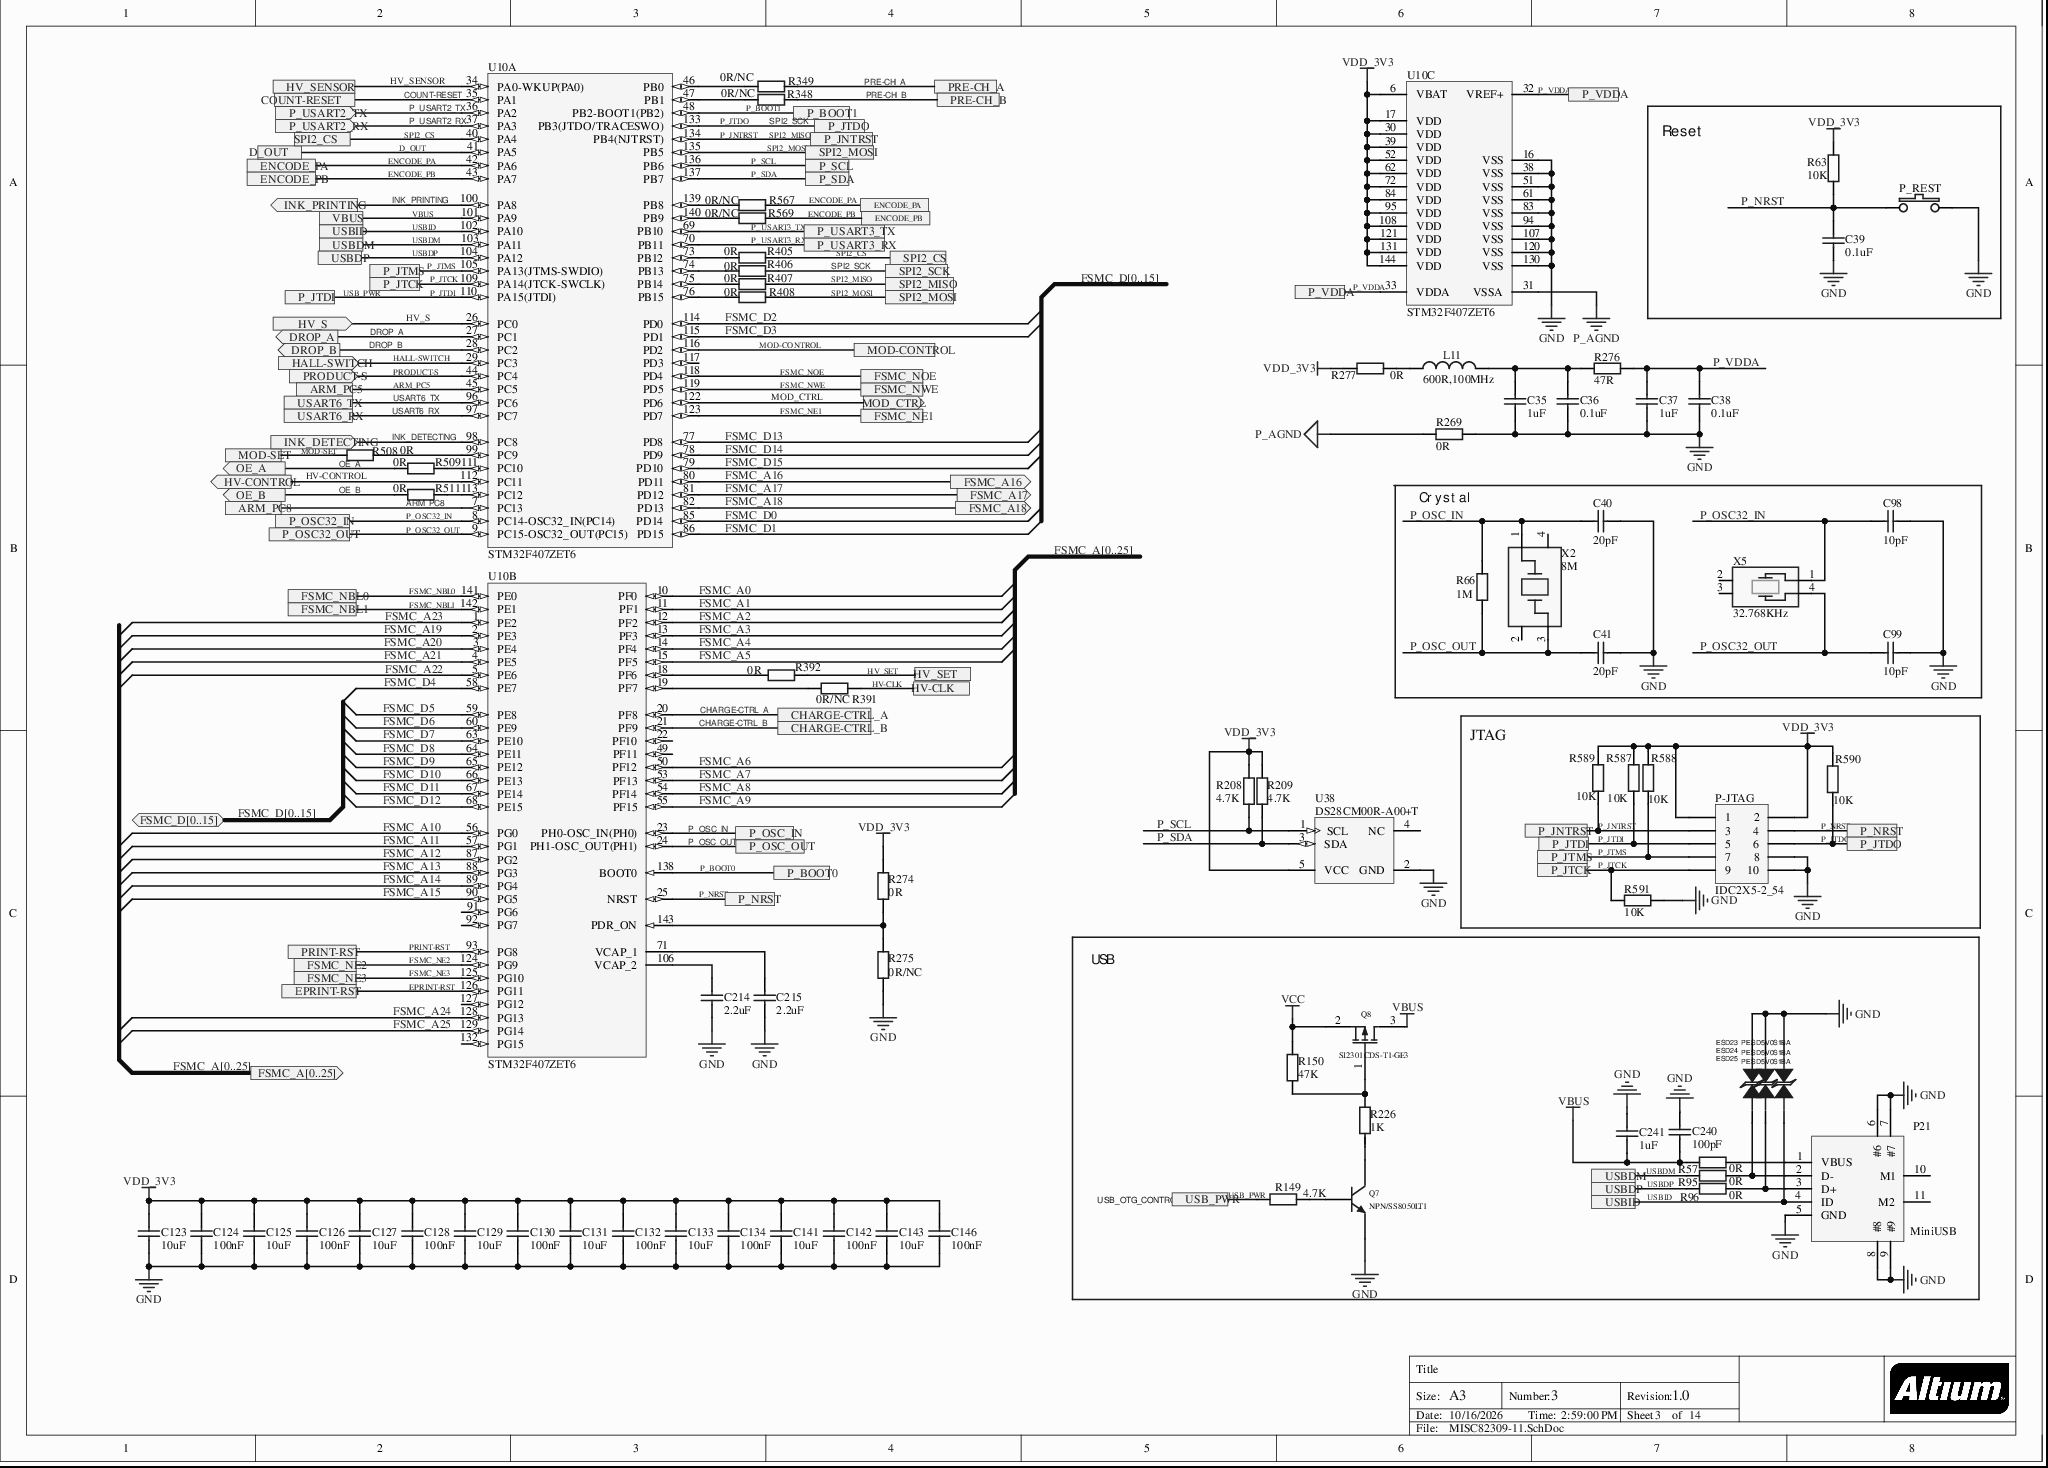
[diagram p0: MISC82309-11.SchDoc]
# Altium project MISC82309-16.PrjPcb (part 2 of 6)
## Sheet MISC82309-11.SchDoc (continued)
### Nets (continued)
ARM_PC5: U10.45(PC5) ; port ARM_PC5
ARM_PC8: U10.7(PC13) ; port ARM_PC8
CHARGE-CTRL_A: U10.20(PF8) ; port CHARGE-CTRL_A
CHARGE-CTRL_B: U10.21(PF9) ; port CHARGE-CTRL_B
COUNT-RESET: U10.35(PA1) ; port COUNT-RESET
D_OUT: U10.41(PA5) ; port D_OUT
DROP_A: U10.27(PC1) ; port DROP_A
DROP_B: U10.28(PC2) ; port DROP_B
ENCODE_PA: R567.2 U10.42(PA6) ; port ENCODE_PA
ENCODE_PB: R569.2 U10.43(PA7) ; port ENCODE_PB
EPRINT-RST: U10.126(PG11) ; port EPRINT-RST
FSMC_A0: U10.10(PF0)
FSMC_A1: U10.11(PF1)
FSMC_A2: U10.12(PF2)
FSMC_A3: U10.13(PF3)
FSMC_A4: U10.14(PF4)
FSMC_A5: U10.15(PF5)
FSMC_A6: U10.50(PF12)
FSMC_A7: U10.53(PF13)
FSMC_A8: U10.54(PF14)
FSMC_A9: U10.55(PF15)
FSMC_A10: U10.56(PG0)
FSMC_A11: U10.57(PG1)
FSMC_A12: U10.87(PG2)
FSMC_A13: U10.88(PG3)
FSMC_A14: U10.89(PG4)
FSMC_A15: U10.90(PG5)
FSMC_A16: U10.80(PD11) ; port FSMC_A16
FSMC_A17: U10.81(PD12) ; port FSMC_A17
FSMC_A18: U10.82(PD13) ; port FSMC_A18
FSMC_A19: U10.2(PE3)
FSMC_A20: U10.3(PE4)
FSMC_A21: U10.4(PE5)
FSMC_A22: U10.5(PE6)
FSMC_A23: U10.1(PE2)
FSMC_A24: U10.128(PG13)
FSMC_A25: U10.129(PG14)
FSMC_D0: U10.85(PD14)
FSMC_D1: U10.86(PD15)
FSMC_D2: U10.114(PD0)
FSMC_D3: U10.115(PD1)
FSMC_D4: U10.58(PE7)
FSMC_D5: U10.59(PE8)
FSMC_D6: U10.60(PE9)
FSMC_D7: U10.63(PE10)
FSMC_D8: U10.64(PE11)
FSMC_D9: U10.65(PE12)
FSMC_D10: U10.66(PE13)
FSMC_D11: U10.67(PE14)
FSMC_D12: U10.68(PE15)
FSMC_D13: U10.77(PD8)
FSMC_D14: U10.78(PD9)
FSMC_D15: U10.79(PD10)
FSMC_NBL0: U10.141(PE0) ; port FSMC_NBL0
FSMC_NBL1: U10.142(PE1) ; port FSMC_NBL1
FSMC_NE1: U10.123(PD7) ; port FSMC_NE1
FSMC_NE2: U10.124(PG9) ; port FSMC_NE2
FSMC_NE3: U10.125(PG10) ; port FSMC_NE3
FSMC_NOE: U10.118(PD4) ; port FSMC_NOE
FSMC_NWE: U10.119(PD5) ; port FSMC_NWE
HALL-SWITCH: U10.29(PC3) ; port HALL-SWITCH
HV-CLK: R391.2 ; port HV-CLK
HV-CONTROL: U10.112(PC11) ; port HV-CONTROL
HV_S: U10.26(PC0) ; port HV_S
HV_SENSOR: U10.34(PA0-WKUP(PA0)) ; port HV_SENSOR
HV_SET: R392.2 ; port HV_SET
INK_DETECTING: U10.98(PC8) ; port INK_DETECTING
INK_PRINTING: U10.100(PA8) ; port INK_PRINTING
MOD-CONTROL: U10.116(PD2) ; port MOD-CONTROL
MOD-SET: R508.2 ; port MOD-SET
MOD_CTRL: U10.122(PD6) ; port MOD_CTRL
OE_A: R509.1 ; port OE_A
OE_B: R511.1 ; port OE_B
P_BOOT0: U10.138(BOOT0) ; port P_BOOT0
P_BOOT1: U10.48(PB2-BOOT1(PB2)) ; port P_BOOT1
P_JNTRST: P-JTAG.3 R407.2 R589.1 U10.134(PB4(NJTRST)) ; port P_JNTRST, port SPI2_MISO  [also labelled SPI2_MISO]
P_JTCK: P-JTAG.9 R591.2 U10.109(PA14(JTCK-SWCLK)) ; port P_JTCK
P_JTDI: P-JTAG.5 R149.1 R587.1 U10.110(PA15(JTDI)) ; port USB_PWR, port P_JTDI  [also labelled USB_PWR]
P_JTDO: P-JTAG.6 R406.2 R590.1 U10.133(PB3(JTDO/TRACESWO)) ; port P_JTDO, port SPI2_SCK  [also labelled SPI2_SCK]
P_JTMS: P-JTAG.7 R588.1 U10.105(PA13(JTMS-SWDIO)) ; port P_JTMS
P_NRST: C39.2 P-JTAG.4 P_REST.1 R63.2 U10.25(NRST) ; port P_NRST
P_OSC32_IN: C98.2 U10.8(PC14-OSC32_IN(PC14)) X5.1 ; port P_OSC32_IN
P_OSC32_OUT: C99.2 U10.9(PC15-OSC32_OUT(PC15)) X5.4 ; port P_OSC32_OUT
P_OSC_IN: C40.2 R66.1 U10.23(PH0-OSC_IN(PH0)) X2.1 ; port P_OSC_IN
P_OSC_OUT: C41.2 R66.2 U10.24(PH1-OSC_OUT(PH1)) X2.3 ; port P_OSC_OUT
P_SCL: R208.2 U10.136(PB6) U38.1(SCL) ; port P_SCL
P_SDA: R209.2 U10.137(PB7) U38.3(SDA) ; port P_SDA
P_USART2_RX: U10.37(PA3) ; port P_USART2_RX
P_USART2_TX: U10.36(PA2) ; port P_USART2_TX
P_USART3_RX: U10.70(PB11) ; port P_USART3_RX
P_USART3_TX: U10.69(PB10) ; port P_USART3_TX
P_VDDA: C37.2 C38.2 R276.2 U10.32(VREF+) U10.33(VDDA) ; port P_VDDA
PRE-CH_A: R349.2 ; port PRE-CH_A
PRE-CH_B: R348.2 ; port PRE-CH_B
PRINT-RST: U10.93(PG8) ; port PRINT-RST
PRODUCT-S: U10.44(PC4) ; port PRODUCT-S
SPI2_CS: R405.2 U10.40(PA4) ; port SPI2_CS
SPI2_MOSI: R408.2 U10.135(PB5) ; port SPI2_MOSI
USART6_RX: U10.97(PC7) ; port USART6_RX
USART6_TX: U10.96(PC6) ; port USART6_TX
USBDM: R95.2 U10.103(PA11) ; port USBDM
USBDP: R96.2 U10.104(PA12) ; port USBDP
USBID: ESD23.1 P21.4(ID) U10.102(PA10) ; port USBID
NetC35_2: C35.2 C36.2 L11.2 R276.1
NetC214_1: C214.1 U10.106(VCAP_2)
NetC215_1: C215.1 U10.71(VCAP_1)
NetESD24_1: ESD24.1 P21.2(D-) R95.1
NetESD25_1: ESD25.1 P21.3(D+) R96.1
NetL11_1: L11.1 R277.2
NetP21_1: P21.1(VBUS) R57.1
NetQ7_1: Q7.1(B) R149.2
NetQ7_3: Q7.3(C) R226.2
NetQ8_1: Q8.1(G) R150.1 R226.1
NetR274_1: R274.1 R275.2 U10.143(PDR_ON)
NetR348_1: R348.1 U10.47(PB1)
NetR349_1: R349.1 U10.46(PB0)
NetR391_1: R391.1 U10.19(PF7)
NetR392_1: R392.1 U10.18(PF6)
NetR405_1: R405.1 U10.73(PB12)
NetR406_1: R406.1 U10.74(PB13)
NetR407_1: R407.1 U10.75(PB14)
NetR408_1: R408.1 U10.76(PB15)
NetR508_1: R508.1 U10.99(PC9)
NetR509_2: R509.2 U10.111(PC10)
NetR511_2: R511.2 U10.113(PC12)
NetR567_1: R567.1 U10.139(PB8)
NetR569_1: R569.1 U10.140(PB9)

Not connected (* = marked no-connect by the designer): P21 10(M1) 11(M2); P_REST 5 6; U10 22(PF10) 49(PF11) 91(PG6) 92(PG7) 117(PD3) 127(PG12) 132(PG15); U38 4(NC); X2 2 4; X5 2 3

### Buses and harness runs
bus FSMC_A[0..25]
bus FSMC_A[0..25] = port FSMC_A[0..25]
bus FSMC_D[0..15]
bus FSMC_D[0..15] = port FSMC_D[0..15]

### Notes on the sheet
- USB_OTG_CONTROL
- Title
- Size:
- Date:
- A3
- Number:
- Time:
- Revision:
- Sheet
- of
- File:

### Library data of the parts
C35-C38 C214 C215 = CAP_0805: Capacitor
  C35 C37: value: 1uF
  C36 C38: value: 0.1uF
  C214 C215: value: 2.2uF
C39 = CAP_1206: Capacitor; value: 0.1uF
C40 C41 C98 C99 C123-C134 C141-C143 C146 = CAP_1206: Capacitor; value: 0.1uF
C240 C241 = CAP_0603: Capacitor
  C240: value: 100pF
  C241: value: 1uF
ESD23-ESD25 = DIODE_TVS_BI-DIR: TVS,BIDIRECTION,5V,RENESAS PROJECT; Manufacturer: NXP; Part_Number: ESDEMI44; SMT_OPTION: YES; Lib_from: MIKE; PACKAGE: SOD882; Manufacturer_Part_Number: PESD5V0S1BA; Description_2: TVS,BIDIRECTION,5V,RENESAS PROJECT; PCB DECAL: SOD323
L11 = Inductor: value: 600R,100MHz
P21 = USB_Slave
P-JTAG = HEAD2X5-2_54
Q7 = NPN: YFLZVQMB: MB4A050S1; AIEP: 43; NRXQ: Transistor; GGULWYUT: SMD NPN transistor, 1.5A, 25V, 0.3W, Ft=100MHZ, Hfe range 120-350; BSHU: SOT-23; ZJYF: PCS; TQWQXLGC: Sunlord; DWCHAXEP: SS8050LT1; PCB DECAL: SOT-23-3; Value: NPN/SS8050LT1; Comment_1: NPN
Q8 = SI2301: MOSFET; YFLZVQMB: MB4E23010; GGULWYUT: SMD PMOS, -20V,-3.1A,1.6W, on-resistance 112mΩ, Qg typical 3.3nC; TQWQXLTW: VISAY; DWCHAXEP: SI2301CDS-T1-GE3; YQWWAXEP: *; PCB DECAL: SOT-23; Comment_1: SI2301
R57 R95 R96 R150 R226 R274 R275 R348 R349 R391 R392 R405-R408 R508 R509 R511 R567 R569 = Res_0603: Res
  R57 R95 R96 R274 R392 R405-R408 R508 R509 R511: value: 0R
  R150: value: 47K
  R226: value: 1K
  R275 R348 R349 R391 R567 R569: value: 0R/NC
R63 R208 R209 = Res2: Resistor; Published: 8-Jun-2000; LatestRevisionDate: 17-Jul-2002; LatestRevisionNote: Re-released for DXP Platform.; PackageReference: AXIAL-0.4; Publisher: Altium Limited
  R63: Value: 10K
  R208 R209: Value: 4.7K
R66 = Res2: Resistor; Value: 10K; Published: 8-Jun-2000; LatestRevisionDate: 17-Jul-2002; LatestRevisionNote: Re-released for DXP Platform.; PackageReference: AXIAL-0.4; Publisher: Altium Limited
R149 = Res2: Resistor; Value: 1K; Published: 8-Jun-2000; LatestRevisionDate: 17-Jul-2002; LatestRevisionNote: Re-released for DXP Platform.; PackageReference: AXIAL-0.4; Publisher: Altium Limited
R269 R276 R277 = Res_0805: Res
  R269 R277: value: 0R
  R276: value: 47R
R587-R591 = Res: value: 10K
U10 = STM32F407ZET6: ARM Cortex-M4 32-bit MCU+FPU, 210 DMIPS, 512 kB Flash, 192 kB Internal RAM, 114 I/Os, 144-pin LQFP, -40 to 85 degC, Tray; Manufacturer: STMicroelectronics; D/A Converter: 2x12-bit; FLASH Size (Prog) (kB): 512; I/Os (High Current): 114; Internal RAM Size (kB): 192; Operating Frequency(F) (Processor speed) (MHz): 168; Supply Voltage(Vcc) max (V): 3.6; Supply Voltage(Vcc) min (V): 1.8; DatasheetVersion: Rev. 4; PackageVersion: Rev. 4, 06/2013; PackageReference: LQFP144; PackageDescription: 144-Pin Low Profile Quad Flat Package, 20 x 20 mm Body, 0.5 mm Pitch; Supplier 1: Digi-Key; Supplier Part Number 1: 497-11903-ND; Supplier 2: Farnell; Supplier Part Number 2: 2215229; Supplier 3: Newark; Supplier Part Number 3: 46W2203; Supplier 4: Newark; Supplier Part Number 4: 87T3795; Supplier 5: Mouser; Supplier Part Number 5: 511-STM32F407ZET6; Core: ARM Cortex-M4; Packing: Tray; Mounting Technology: Surface Mount; PartNumber: STM32F407ZET6; ComponentLink1Description: Manufacturer URL; ComponentLink1URL: http://www.st.com/web/en/home.html; ComponentLink2Description: Datasheet; ComponentLink2URL: http://www.st.com/st-web-ui/static/active/en/resource/technical/document/datasheet/DM00037051.pdf; ComponentLink3Description: Package Specification; ComponentLink3URL: http://www.st.com/st-web-ui/static/active/en/resource/technical/document/datasheet/DM00037051.pdf
U38 = DS28CM00R-A00+T: I睠/SMBus Silicon Serial Number, 5-pin SOT23, -40?to + 85?C, Pb-Free, Tape and Reel; DatasheetVersion: 1/11/2006; PackageVersion: revF, 2006; PackageReference: U5+1; PackageDescription: 5-Pin Small-Outline Transistor Package, 0.95 mm Pitch, 2.8 mm Lead Span, SOT-23, Pb-Free; Code_JEDEC: MO-178AA; ComponentLink1Description: Manufacturer URL; ComponentLink1URL: www.maxim-ic.com; ComponentLink2Description: Datasheet; ComponentLink2URL: http://datasheets.maxim-ic.com/en/ds/DS28CM00.pdf
X2 = CRYSTAL-SMD4: value: SMD5032_8MHZ_4pin
X5 = CRYSTAL-SMD4A: value: 晶体SSP-T7-F32.768KHZ

## Sheet MISC82309-10.SchDoc
size A3; DocumentNumber: 4; Revision: 1.0; SheetNumber: 4; SheetTotal: 14
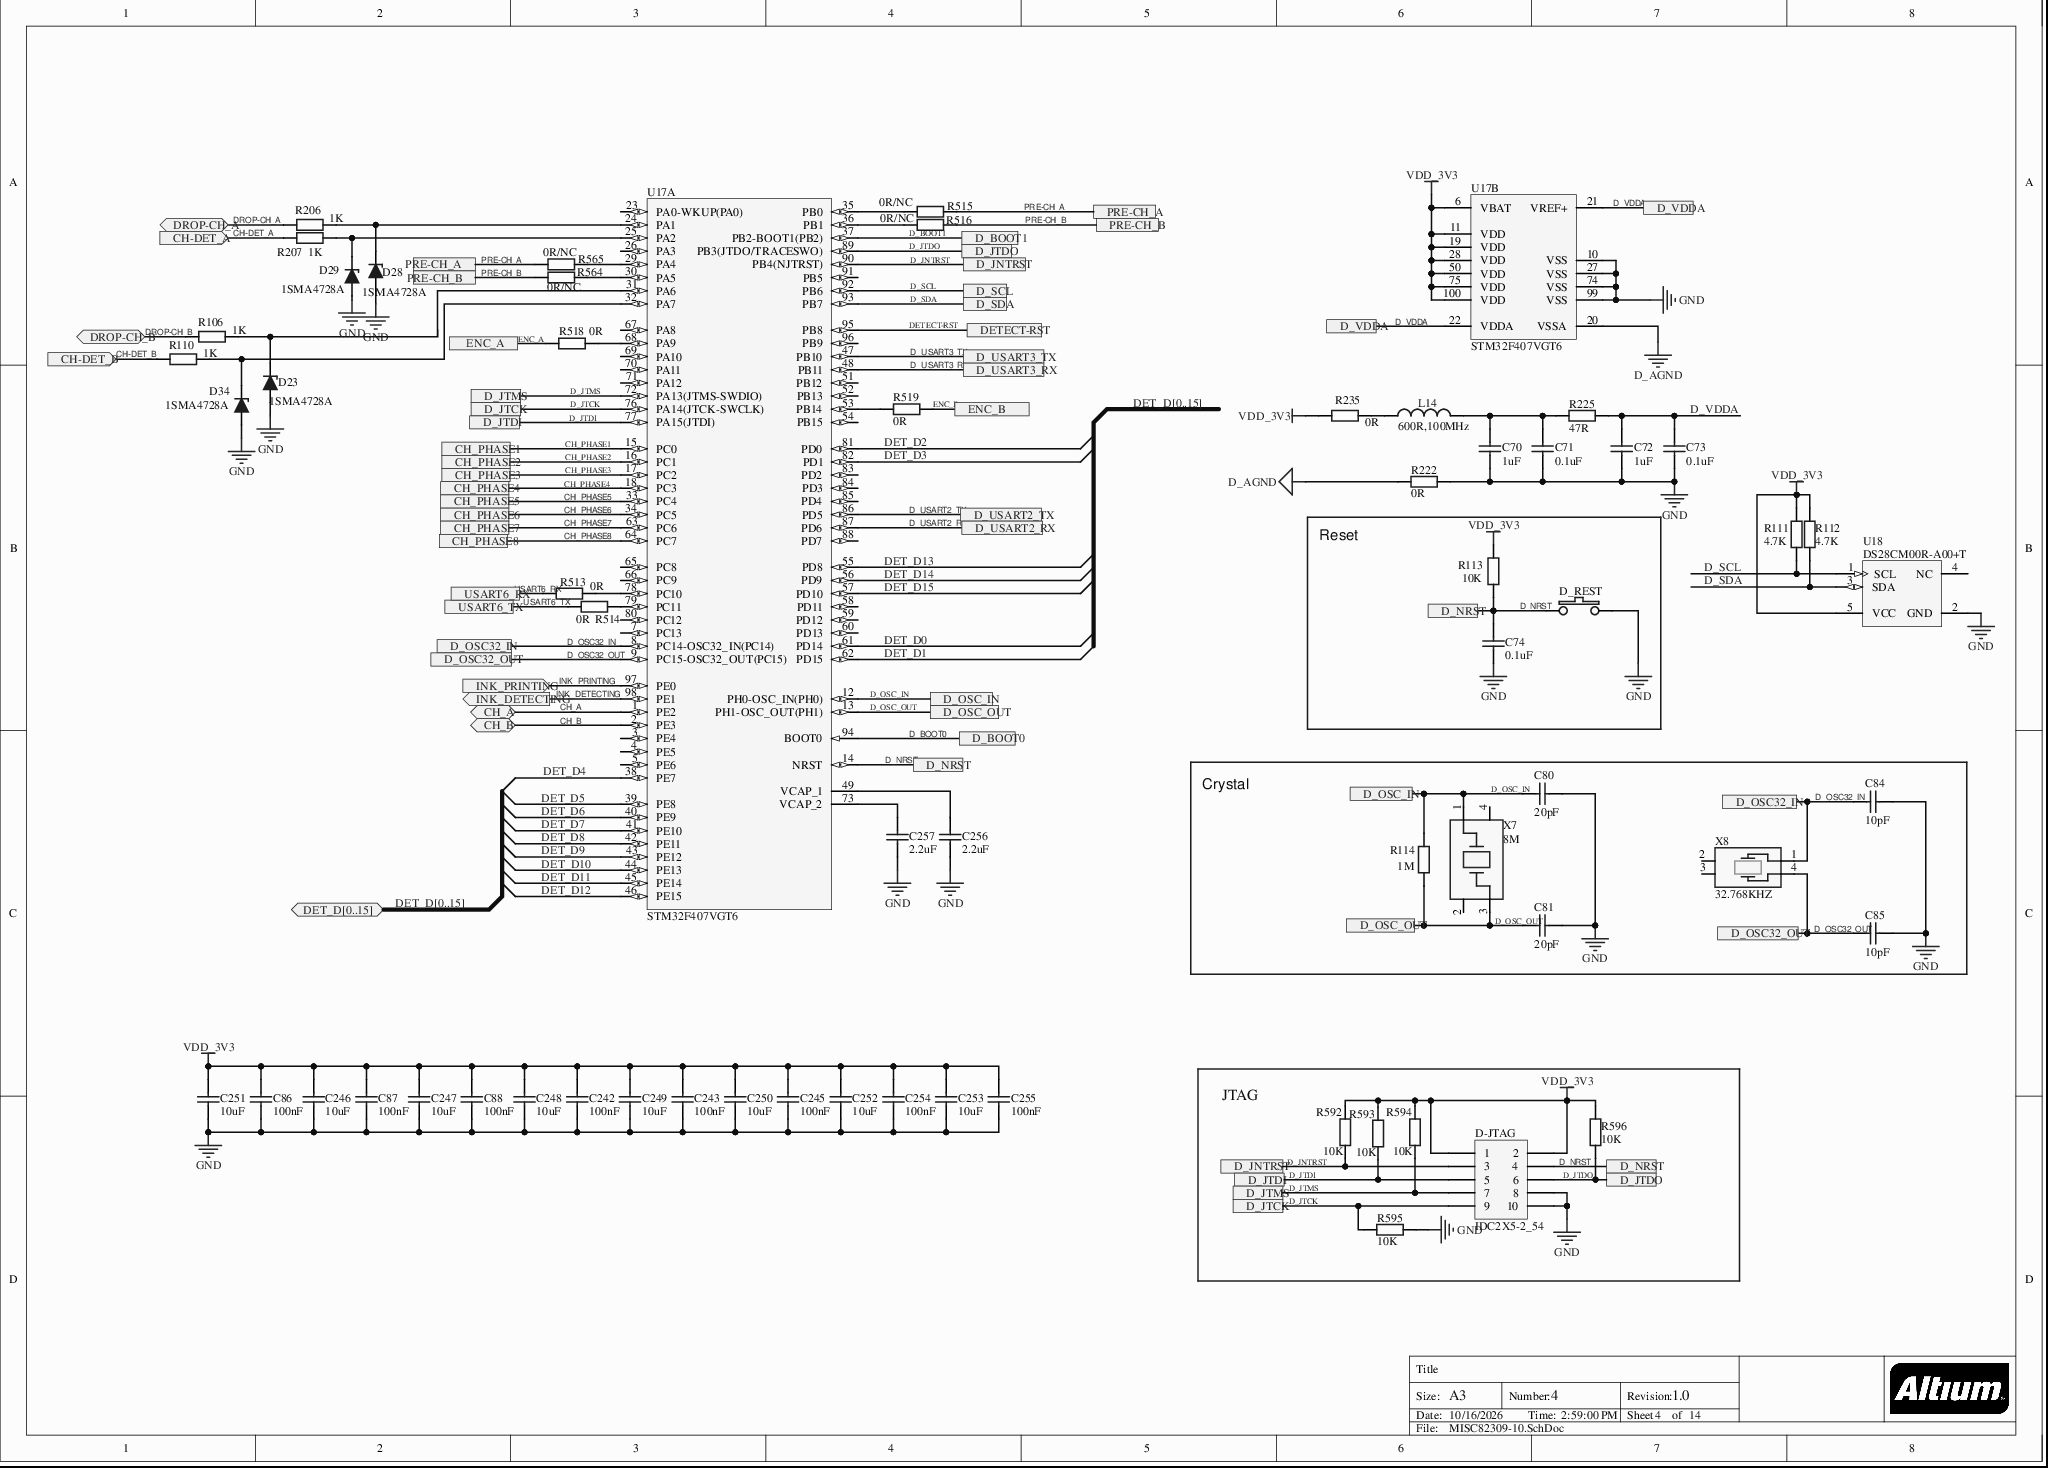
[diagram p1: MISC82309-10.SchDoc]

### Parts
C70  1uF  [CAP_0805]
C71  0.1uF  [CAP_0805]
C72  1uF  [CAP_0805]
C73  0.1uF  [CAP_0805]
C74  0.1uF  [C0603]
C80  20pF  [C0603]
C81  20pF  [C0603]
C84  10pF  [C0603]
C85  10pF  [C0603]
C86  100nF  [C0805]
C87  100nF  [C0805]
C88  100nF  [C0805]
C242  100nF  [C0805]
C243  100nF  [C0805]
C245  100nF  [C0805]
C246  10uF  [C0805]
C247  10uF  [C0805]
C248  10uF  [C0805]
C249  10uF  [C0805]
C250  10uF  [C0805]
C251  10uF  [C0805]
C252  10uF  [C0805]
C253  10uF  [C0805]
C254  100nF  [C0805]
C255  100nF  [C0805]
C256  2.2uF  [CAP_0805]
C257  2.2uF  [CAP_0805]
D23  1SMA4728A  [DO-214AC]
D28  1SMA4728A  [DO-214AC]
D29  1SMA4728A  [DO-214AC]
D34  1SMA4728A  [DO-214AC]
D-JTAG  IDC2X5-2_54  [IDC2X5-2_54]
D_REST  SW  [SW-6X3X2.5]  (value not drawn)
L14  600R,100MHz  [R0805]
R106  1K  [R1206]
R110  1K  [R1206]
R111  4.7K  [R0603]
R112  4.7K  [R0603]
R113  10K  [R0603]
R114  1M  [R0603]
R206  1K  [R1206]
R207  1K  [R1206]
R222  0R  [R0805]
R225  47R  [R0805]
R235  0R  [R0805]
R513  0R  [RES_0603]
R514  0R  [RES_0603]
R515  0R/NC  [RES_0603]
R516  0R/NC  [RES_0603]
R518  0R  [RES_0603]
R519  0R  [RES_0603]
R564  0R/NC  [RES_0603]
R565  0R/NC  [RES_0603]
R592  10K  [R0603]
R593  10K  [R0603]
R594  10K  [R0603]
R595  10K  [R0603]
R596  10K  [R0603]
U17  STM32F407VGT6  [LQFP100_N]  (parts A,B of 2)
U18  DS28CM00R-A00+T  [U5+1_N]
X7  8M  [SMD5032]
X8  32.768KHZ  [Y_XTAL_T7]

### Blocks framed on the sheet
Reset: C74 D_REST R113
Crystal: C80 C81 C84 C85 R114 X7 X8
JTAG: D-JTAG R592-R596

### Ports
CH-DET_A (in), CH-DET_B (in), CH_A (bidir), CH_B (bidir), CH_PHASE1, CH_PHASE2, CH_PHASE3, CH_PHASE4, CH_PHASE5, CH_PHASE6, CH_PHASE7, CH_PHASE8, D_BOOT0, D_BOOT1, D_JNTRST, D_JTCK, D_JTDI, D_JTDO, D_JTMS, D_NRST, D_OSC32_IN, D_OSC32_OUT, D_OSC_IN, D_OSC_OUT, D_SCL, D_SDA, D_USART2_RX, D_USART2_TX, D_USART3_RX, D_USART3_TX, D_VDDA, DET_D[0..15] (bidir), DETECT-RST, DROP-CH_A (bidir), DROP-CH_B (bidir), ENC_A, ENC_B, INK_DETECTING (out), INK_PRINTING (in), PRE-CH_A, PRE-CH_B, USART6_RX, USART6_TX

### Nets
D_AGND: R222.1 U17.20(VSSA)
GND: C70.1 C71.1 C72.1 C73.1 C74.1 C80.1 C81.1 C84.1 C85.1 C86.1 C87.1 C88.1 C242.1 C243.1 C245.1 C246.1 C247.1 C248.1 C249.1 C250.1 C251.1 C252.1 C253.1 C254.1 C255.1 C256.2 C257.2 D23.1 D28.1 D29.1 D34.1 D-JTAG.8 D-JTAG.10 D_REST.2 R222.2 R595.1 U17.10(VSS) U17.27(VSS) U17.74(VSS) U17.99(VSS) U18.2(GND)
VDD_3V3: C86.2 C87.2 C88.2 C242.2 C243.2 C245.2 C246.2 C247.2 C248.2 C249.2 C250.2 C251.2 C252.2 C253.2 C254.2 C255.2 D-JTAG.1 D-JTAG.2 R111.1 R112.1 R113.1 R235.1 R592.2 R593.2 R594.2 R596.1 U17.6(VBAT) U17.11(VDD) U17.19(VDD) U17.28(VDD) U17.50(VDD) U17.75(VDD) U17.100(VDD) U18.5(VCC)
CH-DET_A: R207.1 ; port CH-DET_A
CH-DET_B: R110.1 ; port CH-DET_B
CH_A: U17.1(PE2) ; port CH_A
CH_B: U17.2(PE3) ; port CH_B
CH_PHASE1: U17.15(PC0) ; port CH_PHASE1
CH_PHASE2: U17.16(PC1) ; port CH_PHASE2
CH_PHASE3: U17.17(PC2) ; port CH_PHASE3
CH_PHASE4: U17.18(PC3) ; port CH_PHASE4
CH_PHASE5: U17.33(PC4) ; port CH_PHASE5
CH_PHASE6: U17.34(PC5) ; port CH_PHASE6
CH_PHASE7: U17.63(PC6) ; port CH_PHASE7
CH_PHASE8: U17.64(PC7) ; port CH_PHASE8
D_BOOT0: U17.94(BOOT0) ; port D_BOOT0
D_BOOT1: U17.37(PB2-BOOT1(PB2)) ; port D_BOOT1
D_JNTRST: D-JTAG.3 R592.1 U17.90(PB4(NJTRST)) ; port D_JNTRST
D_JTCK: D-JTAG.9 R595.2 U17.76(PA14(JTCK-SWCLK)) ; port D_JTCK
D_JTDI: D-JTAG.5 R593.1 U17.77(PA15(JTDI)) ; port D_JTDI
D_JTDO: D-JTAG.6 R596.2 U17.89(PB3(JTDO/TRACESWO)) ; port D_JTDO
D_JTMS: D-JTAG.7 R594.1 U17.72(PA13(JTMS-SWDIO)) ; port D_JTMS
D_NRST: C74.2 D-JTAG.4 D_REST.1 R113.2 U17.14(NRST) ; port D_NRST
D_OSC32_IN: C84.2 U17.8(PC14-OSC32_IN(PC14)) X8.1 ; port D_OSC32_IN
D_OSC32_OUT: C85.2 U17.9(PC15-OSC32_OUT(PC15)) X8.4 ; port D_OSC32_OUT
D_OSC_IN: C80.2 R114.1 U17.12(PH0-OSC_IN(PH0)) X7.1 ; port D_OSC_IN
D_OSC_OUT: C81.2 R114.2 U17.13(PH1-OSC_OUT(PH1)) X7.3 ; port D_OSC_OUT
D_SCL: R111.2 U17.92(PB6) U18.1(SCL) ; port D_SCL
D_SDA: R112.2 U17.93(PB7) U18.3(SDA) ; port D_SDA
D_USART2_RX: U17.87(PD6) ; port D_USART2_RX
D_USART2_TX: U17.86(PD5) ; port D_USART2_TX
D_USART3_RX: U17.48(PB11) ; port D_USART3_RX
D_USART3_TX: U17.47(PB10) ; port D_USART3_TX
D_VDDA: C72.2 C73.2 R225.2 U17.21(VREF+) U17.22(VDDA) ; port D_VDDA
DET_D0: U17.61(PD14)
DET_D1: U17.62(PD15)
DET_D2: U17.81(PD0)
DET_D3: U17.82(PD1)
DET_D4: U17.38(PE7)
DET_D5: U17.39(PE8)
DET_D6: U17.40(PE9)
DET_D7: U17.41(PE10)
DET_D8: U17.42(PE11)
DET_D9: U17.43(PE12)
DET_D10: U17.44(PE13)
DET_D11: U17.45(PE14)
DET_D12: U17.46(PE15)
DET_D13: U17.55(PD8)
DET_D14: U17.56(PD9)
DET_D15: U17.57(PD10)
DETECT-RST: U17.95(PB8) ; port DETECT-RST
DROP-CH_A: R206.1 ; port DROP-CH_A
DROP-CH_B: R106.1 ; port DROP-CH_B
ENC_A: R518.2 ; port ENC_A
ENC_B: R519.2 ; port ENC_B
INK_DETECTING: U17.98(PE1) ; port INK_DETECTING
INK_PRINTING: U17.97(PE0) ; port INK_PRINTING
PRE-CH_A: R515.2 R565.1 ; port PRE-CH_A
PRE-CH_B: R516.2 R564.1 ; port PRE-CH_B
USART6_RX: R513.2 ; port USART6_RX
USART6_TX: R514.2 ; port USART6_TX
NetC70_2: C70.2 C71.2 L14.2 R225.1
NetC256_1: C256.1 U17.49(VCAP_1)
NetC257_1: C257.1 U17.73(VCAP_2)
NetD23_2: D23.2 R106.2 U17.31(PA6)
NetD28_2: D28.2 R206.2 U17.24(PA1)
NetD29_2: D29.2 R207.2 U17.25(PA2)
NetD34_2: D34.2 R110.2 U17.32(PA7)
NetL14_1: L14.1 R235.2
NetR513_1: R513.1 U17.78(PC10)
NetR514_1: R514.1 U17.79(PC11)
NetR515_1: R515.1 U17.35(PB0)
NetR516_1: R516.1 U17.36(PB1)
NetR518_1: R518.1 U17.68(PA9)
NetR519_1: R519.1 U17.53(PB14)
NetR564_2: R564.2 U17.30(PA5)
NetR565_2: R565.2 U17.29(PA4)

Not connected (* = marked no-connect by the designer): D_REST 5 6; U17 3(PE4) 4(PE5) 5(PE6) 7(PC13) 23(PA0-WKUP(PA0)) 26(PA3) 51(PB12) 52(PB13) 54(PB15) 58(PD11) 59(PD12) 60(PD13) 65(PC8) 66(PC9) 67(PA8) 69(PA10) 70(PA11) 71(PA12) 80(PC12) 83(PD2) 84(PD3) 85(PD4) 88(PD7) 91(PB5) 96(PB9); U18 4(NC); X7 2 4; X8 2 3

### Buses and harness runs
bus DET_D[0..15]
bus DET_D[0..15] = port DET_D[0..15]

### Notes on the sheet
- Labels drawn without touching a wire or pin: USART6_RX
- Title
- Size:
- Date:
- A3
- Number:
- Time:
- Revision:
- Sheet
- of
- File:

### Library data of the parts
C70-C73 C256 C257 = CAP_0805: Capacitor
  C70 C72: value: 1uF
  C71 C73: value: 0.1uF
  C256 C257: value: 2.2uF
C74 = CAP_1206: Capacitor; value: 0.1uF
C80 C81 C84-C88 C242 C243 C245-C255 = CAP_1206: Capacitor; value: 0.1uF
D23 D28 D29 D34 = 1SMA4728A: 1SMA4728A 1W 3.3V SMA DO-214AC
D-JTAG = HEAD2X5-2_54
L14 = Inductor: value: 600R,100MHz
R106 R110 R206 R207 R592-R596 = Res
  R106 R110 R206 R207: value: 1K
  R592-R596: value: 10K
R111-R113 = Res2: Resistor; Published: 8-Jun-2000; LatestRevisionDate: 17-Jul-2002; LatestRevisionNote: Re-released for DXP Platform.; PackageReference: AXIAL-0.4; Publisher: Altium Limited
  R111 R112: Value: 4.7K
  R113: Value: 10K
R114 = Res2: Resistor; Value: 10K; Published: 8-Jun-2000; LatestRevisionDate: 17-Jul-2002; LatestRevisionNote: Re-released for DXP Platform.; PackageReference: AXIAL-0.4; Publisher: Altium Limited
R222 R225 R235 = Res_0805: Res
  R222 R235: value: 0R
  R225: value: 47R
R513-R516 R518 R519 R564 R565 = Res_0603: Res
  R513 R514 R518 R519: value: 0R
  R515 R516 R564 R565: value: 0R/NC
U17 = STM32F407VGT6: ARM Cortex-M4 32-bit MCU+FPU, 210 DMIPS, 1024 kB Flash, 192 kB Internal RAM, 82 I/Os, 100-pin LQFP, -40 to 85 degC, Tray; Manufacturer: STMicroelectronics; D/A Converter: 2x12-bit; FLASH Size (Prog) (kB): 1024; I/Os (High Current): 82; Internal RAM Size (kB): 192; Operating Frequency(F) (Processor speed) (MHz): 168; Supply Voltage(Vcc) max (V): 3.6; Supply Voltage(Vcc) min (V): 1.8; DatasheetVersion: Rev. 4; PackageVersion: Rev. 1, 06/2013; PackageReference: LQFP100; PackageDescription: 100-Pin Low Profile Quad Flat Package, 14 x 14 mm Body, 0.5 mm Pitch; Supplier 1: Digi-Key; Supplier Part Number 1: 497-11605-ND; Supplier 2: Farnell; Supplier Part Number 2: 2064368; Supplier 3: Newark; Supplier Part Number 3: 73T2333; Supplier 4: Mouser; Supplier Part Number 4: 511-STM32F407VGT6; Core: ARM Cortex-M4; Packing: Tray; Mounting Technology: Surface Mount; PartNumber: STM32F407VGT6; ComponentLink1Description: Manufacturer URL; ComponentLink1URL: http://www.st.com/web/en/home.html; ComponentLink2Description: Datasheet; ComponentLink2URL: http://www.st.com/st-web-ui/static/active/en/resource/technical/document/datasheet/DM00037051.pdf; ComponentLink3Description: Package Specification; ComponentLink3URL: http://www.st.com/st-web-ui/static/active/en/resource/technical/document/data_brief/DM00071938.pdf
U18 = DS28CM00R-A00+T: I²C/SMBus Silicon Serial Number, 5-pin SOT23, -40?to + 85?C, Pb-Free, Tape and Reel; DatasheetVersion: 1/11/2006; PackageVersion: revF, 2006; PackageReference: U5+1; PackageDescription: 5-Pin Small-Outline Transistor Package, 0.95 mm Pitch, 2.8 mm Lead Span, SOT-23, Pb-Free; Code_JEDEC: MO-178AA; ComponentLink1Description: Manufacturer URL; ComponentLink1URL: www.maxim-ic.com; ComponentLink2Description: Datasheet; ComponentLink2URL: http://datasheets.maxim-ic.com/en/ds/DS28CM00.pdf
X7 = CRYSTAL-SMD4: value: SMD5032_8MHZ_4pin
X8 = CRYSTAL-SMD4A: value: SSP-T7-F32.768KHZ